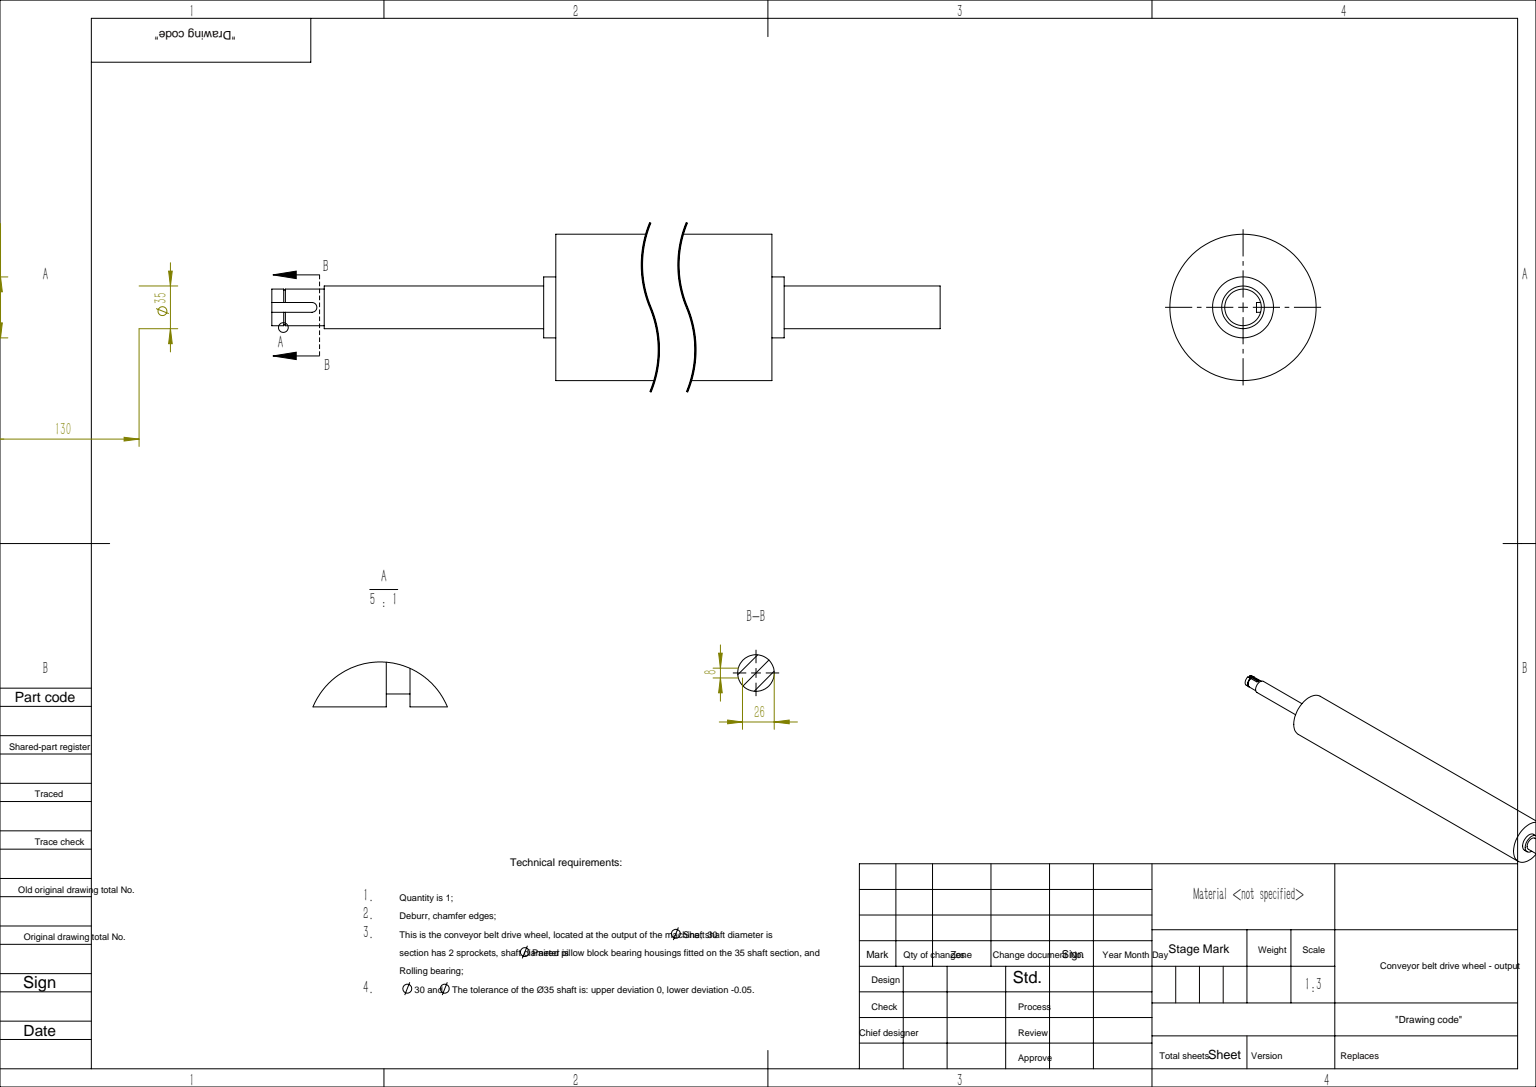
from build123d import *

# Parameters (mm, degrees)
CUT_EXTRUDE_1_DEPTH = 4
CUT_EXTRUDE_START   = -1.3
SKETCH_3_R          = 15
SKETCH_3_R_2        = 14.3
CUT_EXTRUDE_2_DEPTH = 1.3


with BuildPart() as part:
    # 草图1 → 旋转1 (revolve)
    with BuildSketch(Plane.XY, mode=Mode.PRIVATE) as revolve_1_sk:
        Polygon((0, 0), (0, 15), (43, 15), (43, 17.5), (223, 17.5), (223, 25), (233, 25), (233, 60), (1083, 60), (1083, 25), (1093, 25), (1093, 17.5), (1221, 17.5), (1221, 0), align=None)
    revolve(revolve_1_sk.sketch.rotate(Axis((0, 0, 0), (1, 0, 0)), 90), axis=Axis((0, 0, 0), (1, 0, 0)))

    # 草图2 → 切除-拉伸1 (cut)
    with BuildSketch(Plane(origin=(0, 15, 0), x_dir=(1, 0, 0), z_dir=(0, 1, 0))):
        with BuildLine():
            Line((33, 4), (-10, 4))
            Line((-10, 4), (-10, -4))
            Line((-10, -4), (33, -4))
            ThreePointArc((33, -4), (37, 0), (33, 4))
        make_face()
    extrude(amount=-CUT_EXTRUDE_1_DEPTH, mode=Mode.SUBTRACT)

    # 草图3 → 切除-拉伸2 (cut)
    with BuildSketch(Plane.ZY.offset(-9.8).offset(CUT_EXTRUDE_START)):
        Circle(SKETCH_3_R)
        Circle(SKETCH_3_R_2, mode=Mode.SUBTRACT)
    extrude(amount=CUT_EXTRUDE_2_DEPTH, mode=Mode.SUBTRACT)


solid = part.part
